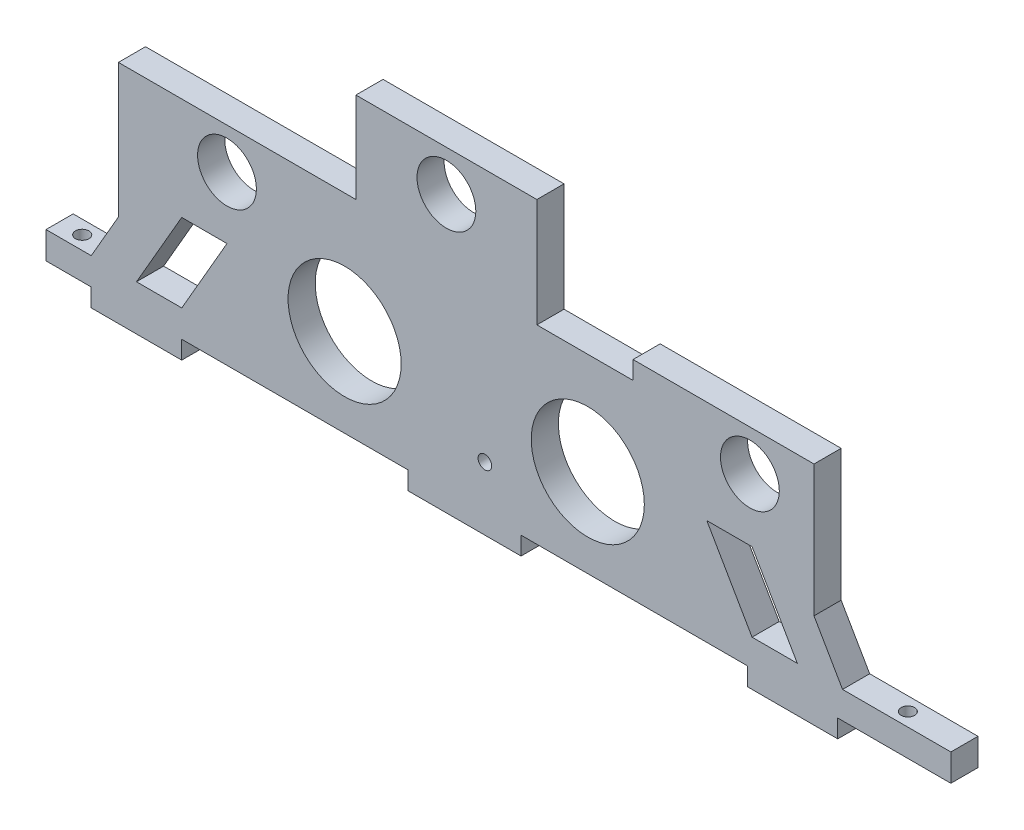
from build123d import *
from build123d.topology import SkipClean

# Parameters (mm, degrees)
SKETCH1_W           = 200
SKETCH1_H           = 45
BOSS_EXTRUDE1_DEPTH = 6
CUT_EXTRUDE1_REACH  = 104.675
SKETCH2_W           = 10
SKETCH2_H           = 3
SKETCH2_W_2         = 50
SKETCH2_W_3         = 25
BOSS_EXTRUDE2_DEPTH = 6
CUT_EXTRUDE2_DEPTH  = 6
CUT_EXTRUDE3_DEPTH  = 6
SKETCH15_R          = 12.5
CUT_EXTRUDE4_DEPTH  = 6
BOSS_EXTRUDE3_DEPTH = 6
SKETCH20_R          = 1.5
CUT_EXTRUDE5_DEPTH  = 111.44568801
SKETCH21_R          = 1.5
CUT_EXTRUDE6_DEPTH  = 117.773284616
SKETCH24_W          = 20
SKETCH24_H          = 6
SKETCH24_W_2        = 25
BOSS_EXTRUDE4_DEPTH = 1
SKETCH25_R          = 6.5
BOSS_EXTRUDE5_DEPTH = 6
SKETCH26_R          = 6.5
CUT_EXTRUDE7_DEPTH  = 111.44568801


with BuildPart() as part:
    # Sketch1 → Boss-Extrude1 (new body)
    with BuildSketch(Plane.XY):
        Rectangle(SKETCH1_W, SKETCH1_H)
    extrude(amount=BOSS_EXTRUDE1_DEPTH)

    # Sketch2 → Cut-Extrude1 (cut, up to next)
    with BuildSketch(Plane.XY.offset(6), mode=Mode.PRIVATE) as cut_extrude1_sk1:
        with Locations((-95, -21)):
            Rectangle(SKETCH2_W, SKETCH2_H)
    cut_extrude1_tool1 = extrude(cut_extrude1_sk1.sketch, amount=-CUT_EXTRUDE1_REACH, mode=Mode.PRIVATE) & part.part
    # Sketch2 → Cut-Extrude1 (cut, up to next)
    with BuildSketch(Plane.XY.offset(6), mode=Mode.PRIVATE) as cut_extrude1_sk2:
        with Locations((-45, -21)):
            Rectangle(SKETCH2_W_2, SKETCH2_H)
    cut_extrude1_tool2 = extrude(cut_extrude1_sk2.sketch, amount=-CUT_EXTRUDE1_REACH, mode=Mode.PRIVATE) & part.part
    # Sketch2 → Cut-Extrude1 (cut, up to next)
    with BuildSketch(Plane.XY.offset(6), mode=Mode.PRIVATE) as cut_extrude1_sk3:
        with Locations((30, -21)):
            Rectangle(SKETCH2_W_2, SKETCH2_H)
    cut_extrude1_tool3 = extrude(cut_extrude1_sk3.sketch, amount=-CUT_EXTRUDE1_REACH, mode=Mode.PRIVATE) & part.part
    # Sketch2 → Cut-Extrude1 (cut, up to next)
    with BuildSketch(Plane.XY.offset(6), mode=Mode.PRIVATE) as cut_extrude1_sk4:
        with Locations((87.5, -21)):
            Rectangle(SKETCH2_W_3, SKETCH2_H)
    cut_extrude1_tool4 = extrude(cut_extrude1_sk4.sketch, amount=-CUT_EXTRUDE1_REACH, mode=Mode.PRIVATE) & part.part
    add(cut_extrude1_tool1.solids().sort_by_distance((-95, -21, 6))[0], mode=Mode.SUBTRACT)
    add(cut_extrude1_tool2.solids().sort_by_distance((-45, -21, 6))[0], mode=Mode.SUBTRACT)
    add(cut_extrude1_tool3.solids().sort_by_distance((30, -21, 6))[0], mode=Mode.SUBTRACT)
    add(cut_extrude1_tool4.solids().sort_by_distance((87.5, -21, 6))[0], mode=Mode.SUBTRACT)

    # Sketch3 → Boss-Extrude2 (add)
    with BuildSketch(Plane.XY.offset(6)):
        with BuildLine():
            Line((-31.5, 42.5), (-31.5, 22.5))
            Line((-31.5, 22.5), (8.5, 22.5))
            Line((8.5, 22.5), (8.5, 42.5))
            Line((8.5, 42.5), (-2, 42.5))
            Line((-2, 42.5), (-2, 37.5))
            Line((-2, 37.5), (-5, 37.5))
            ThreePointArc((-5, 37.5), (-11.5, 31), (-18, 37.5))
            Line((-18, 37.5), (-21, 37.5))
            Line((-21, 37.5), (-21, 42.5))
            Line((-21, 42.5), (-31.5, 42.5))
        make_face()
    extrude(amount=-BOSS_EXTRUDE2_DEPTH)

    # Sketch4 → Cut-Extrude2 (cut)
    with BuildSketch(Plane.XY.offset(6)):
        with BuildLine():
            Line((-53.5, 17.5), (-50.5, 17.5))
            Line((-50.5, 17.5), (-50.5, 22.5))
            Line((-50.5, 22.5), (-69.5, 22.5))
            Line((-69.5, 22.5), (-69.5, 17.5))
            Line((-69.5, 17.5), (-66.5, 17.5))
            ThreePointArc((-66.5, 17.5), (-60, 11), (-53.5, 17.5))
        make_face()
        with BuildLine():
            Line((53, 17.5), (56, 17.5))
            Line((56, 17.5), (56, 22.5))
            Line((56, 22.5), (37, 22.5))
            Line((37, 22.5), (37, 17.5))
            Line((37, 17.5), (40, 17.5))
            ThreePointArc((40, 17.5), (46.5, 11), (53, 17.5))
        make_face()
    extrude(amount=-CUT_EXTRUDE2_DEPTH, mode=Mode.SUBTRACT)

    # Sketch11 → Cut-Extrude3 (cut)
    with BuildSketch(Plane.XY.offset(6)):
        Polygon((-100, -13.5), (-90, -13.5), (-84, -3.107695155), (-84, 22.5), (-100, 22.5), align=None)
        Polygon((100, -13.5), (76.06, -13.5), (69.75, -2.570759404), (69.75, 22.5), (100, 22.5), align=None)
    extrude(amount=-CUT_EXTRUDE3_DEPTH, mode=Mode.SUBTRACT)

    # Sketch15 → Cut-Extrude4 (cut)
    with BuildSketch(Plane.XY.offset(6)):
        with Locations((-34, 0)):
            Circle(SKETCH15_R)
        with Locations((19.75, 0)):
            Circle(SKETCH15_R)
        Polygon((-80, -13.5), (-70, 3.820508076), (-60, 3.820508076), (-69.988315066, -13.5), align=None)
        Polygon((66.06, -13.5), (56.06, 3.820508076), (46.06, 3.820508076), (56.06, -13.5), align=None)
    extrude(amount=-CUT_EXTRUDE4_DEPTH, mode=Mode.SUBTRACT)

    # Sketch19 → Boss-Extrude3 (add)
    with SkipClean():  # the faces are left unmerged after this step: merging them gives an invalid solid
        with BuildSketch(Plane.XY.offset(6)):
            with BuildLine():
                Line((-84, 26.5), (-84, 22.5))
                Line((-84, 22.5), (-69.5, 22.5))
                Line((-69.5, 22.5), (-69.5, 17.5))
                Line((-69.5, 17.5), (-66.5, 17.5))
                ThreePointArc((-66.5, 17.5), (-60, 24), (-53.5, 17.5))
                Line((-53.5, 17.5), (-50.5, 17.5))
                Line((-50.5, 17.5), (-50.5, 22.5))
                Line((-50.5, 22.5), (-31.5, 22.5))
                Line((-31.5, 22.5), (-31.5, 26.5))
                Line((-31.5, 26.5), (-84, 26.5))
            make_face()
            with BuildLine():
                Line((-31.5, 46.5), (-31.5, 42.5))
                Line((-31.5, 42.5), (-21, 42.5))
                Line((-21, 42.5), (-21, 37.5))
                Line((-21, 37.5), (-18, 37.5))
                ThreePointArc((-18, 37.5), (-11.5, 44), (-5, 37.5))
                Line((-5, 37.5), (-2, 37.5))
                Line((-2, 37.5), (-2, 42.5))
                Line((-2, 42.5), (8.5, 42.5))
                Line((8.5, 42.5), (8.5, 46.5))
                Line((8.5, 46.5), (-31.5, 46.5))
            make_face()
            with BuildLine():
                Line((29.75, 26.5), (29.75, 22.5))
                Line((29.75, 22.5), (37, 22.5))
                Line((37, 22.5), (37, 17.5))
                Line((37, 17.5), (40, 17.5))
                ThreePointArc((40, 17.5), (46.5, 24), (53, 17.5))
                Line((53, 17.5), (56, 17.5))
                Line((56, 17.5), (56, 22.5))
                Line((56, 22.5), (69.75, 22.5))
                Line((69.75, 22.5), (69.75, 26.5))
                Line((69.75, 26.5), (29.75, 26.5))
            make_face()
        extrude(amount=-BOSS_EXTRUDE3_DEPTH)

    # Sketch20 → Cut-Extrude5 (cut, through all)
    with SkipClean():  # the faces are left unmerged after this step: merging them gives an invalid solid
        with BuildSketch(Plane(origin=(0, 0, 0), x_dir=(-1, 0, 0), z_dir=(0, 0, -1))):
            with Locations((3, -9.5)):
                Circle(SKETCH20_R)
        extrude(amount=-CUT_EXTRUDE5_DEPTH, mode=Mode.SUBTRACT)

    # Sketch21 → Cut-Extrude6 (cut, through all)
    with SkipClean():  # the faces are left unmerged after this step: merging them gives an invalid solid
        with BuildSketch(Plane(origin=(0, -13.5, 0), x_dir=(1, 0, 0), z_dir=(0, 1, 0))):
            with Locations(Location((87.5, -3, 0), (0, 0, 270))):
                Circle(SKETCH21_R)
            with Locations(Location((-95, -3, 0), (0, 0, 270))):
                Circle(SKETCH21_R)
        extrude(amount=-CUT_EXTRUDE6_DEPTH, mode=Mode.SUBTRACT)

    # Sketch24 → Boss-Extrude4 (add)
    with SkipClean():  # the faces are left unmerged after this step: merging them gives an invalid solid
        with BuildSketch(Plane.XZ.offset(22.5)):
            with Locations((-80, 3)):
                Rectangle(SKETCH24_W, SKETCH24_H)
            with Locations((-7.5, 3)):
                Rectangle(SKETCH24_W_2, SKETCH24_H)
            with Locations((65, 3)):
                Rectangle(SKETCH24_W, SKETCH24_H)
        extrude(amount=BOSS_EXTRUDE4_DEPTH)

    # Sketch25 → Boss-Extrude5 (add)
    with BuildSketch(Plane.XY.offset(6)):
        with Locations((46.5, 17.5)):
            Circle(SKETCH25_R)
        with Locations((-60, 17.5)):
            Circle(SKETCH25_R)
    extrude(amount=-BOSS_EXTRUDE5_DEPTH)

    # Sketch26 → Cut-Extrude7 (cut, through all)
    with BuildSketch(Plane.XY.offset(6)):
        with Locations((55.58, 17.5)):
            Circle(SKETCH26_R)
        with Locations((-60, 17.5)):
            Circle(SKETCH26_R)
    extrude(amount=-CUT_EXTRUDE7_DEPTH, mode=Mode.SUBTRACT)


solid = part.part
